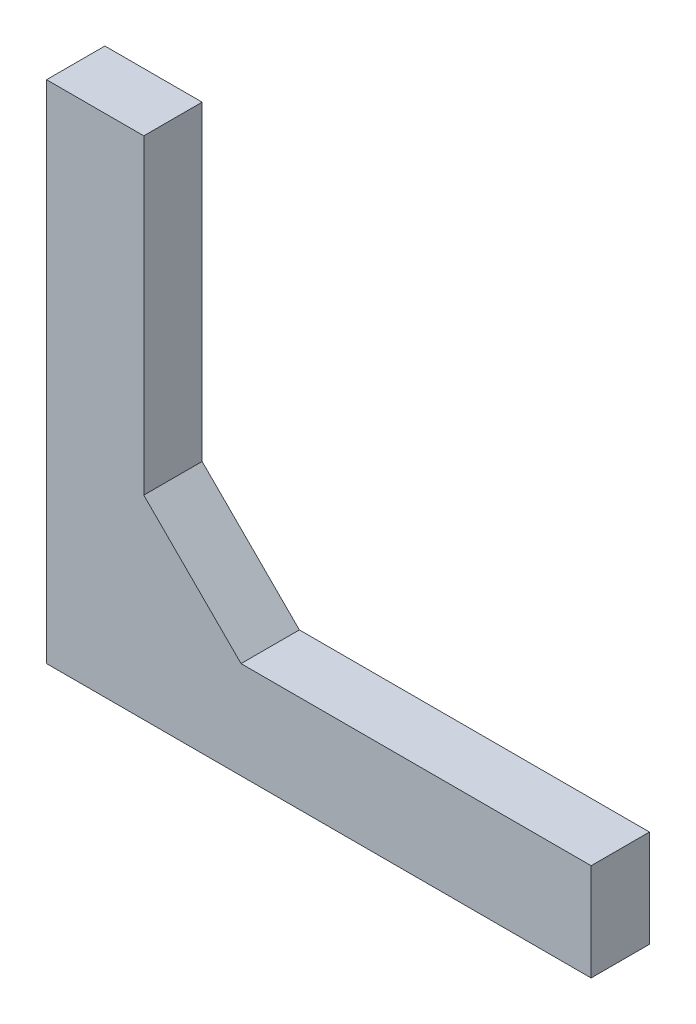
from build123d import *

# Parameters (mm, degrees)
EXTRUDE_1_DEPTH                  = 7.5
HOLE_WIZARD_M6_1_D               = 5
HOLE_WIZARD_M6_1_DEPTH           = 12.5
HOLE_WIZARD_M6_1_TIP             = 1.502151548
HOLE_WIZARD_M6_1_ON_FACE_2_D     = 5
HOLE_WIZARD_M6_1_ON_FACE_2_DEPTH = 12.5
HOLE_WIZARD_M6_1_ON_FACE_2_TIP   = 1.502151548


with BuildPart() as part:
    # 草图1 → 凸台-拉伸1 (new, symmetric)
    with BuildSketch(Plane.XY):
        Polygon((0, 130), (0, 0), (140, 0), (140, 25), (50, 25), (25, 50), (25, 130), align=None)
    extrude(amount=EXTRUDE_1_DEPTH, both=True)

    # M6 螺纹孔1
    with Locations(Plane(origin=(122.5, 0, 0), x_dir=(0, 0, -1), z_dir=(0, -1, 0))):
        with Locations((0, 0), (0, -50), (0, -100)):
            Hole(HOLE_WIZARD_M6_1_D / 2, depth=HOLE_WIZARD_M6_1_DEPTH)
            with Locations((0, 0, -(HOLE_WIZARD_M6_1_DEPTH + HOLE_WIZARD_M6_1_TIP / 2))):  # 118° drill point
                Cone(0, HOLE_WIZARD_M6_1_D / 2, HOLE_WIZARD_M6_1_TIP, mode=Mode.SUBTRACT)

    # M6 螺纹孔1 on face 2
    with Locations(Plane(origin=(0, 30, 0), x_dir=(0, 0, -1), z_dir=(-1, 0, 0))):
        with Locations((0, 0), (0, -45), (0, -90)):
            Hole(HOLE_WIZARD_M6_1_ON_FACE_2_D / 2, depth=HOLE_WIZARD_M6_1_ON_FACE_2_DEPTH)
            with Locations((0, 0, -(HOLE_WIZARD_M6_1_ON_FACE_2_DEPTH + HOLE_WIZARD_M6_1_ON_FACE_2_TIP / 2))):  # 118° drill point
                Cone(0, HOLE_WIZARD_M6_1_ON_FACE_2_D / 2, HOLE_WIZARD_M6_1_ON_FACE_2_TIP, mode=Mode.SUBTRACT)


solid = part.part
